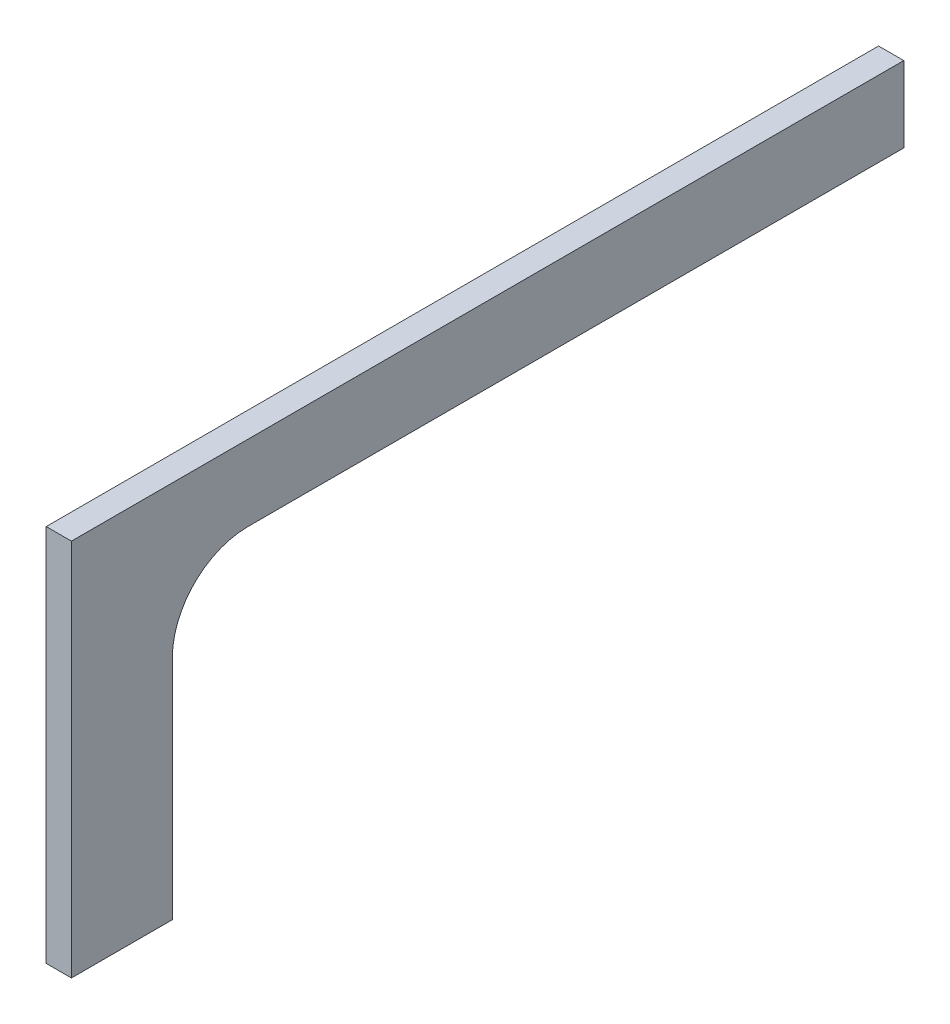
from build123d import *

# Parameters (mm, degrees)
SKETCH_1_W          = 20
SKETCH_1_H          = 300
EXTRUDE_1_DEPTH     = 330
SKETCH_2_W          = 580
SKETCH_2_H          = 240
CUT_EXTRUDE_1_DEPTH = 364.042697213
FILLET_1_R          = 60


with BuildPart() as part:
    # 草图1 → 凸台-拉伸1 (new, symmetric)
    with BuildSketch(Plane.XY):
        Rectangle(SKETCH_1_W, SKETCH_1_H)
    extrude(amount=EXTRUDE_1_DEPTH, both=True)

    # 草图2 → 切除-拉伸1 (cut, through all)
    with BuildSketch(Plane(origin=(10, 0, 0), x_dir=(0, 0, -1), z_dir=(1, 0, 0))):
        with Locations((40, -30)):
            Rectangle(SKETCH_2_W, SKETCH_2_H)
    extrude(amount=-CUT_EXTRUDE_1_DEPTH, mode=Mode.SUBTRACT)

    # 圆角1
    fillet_1_edges = [part.edges().sort_by_distance(p)[0] for p in [
        (0, 90, 250),
    ]]
    fillet(fillet_1_edges, radius=FILLET_1_R)


solid = part.part
